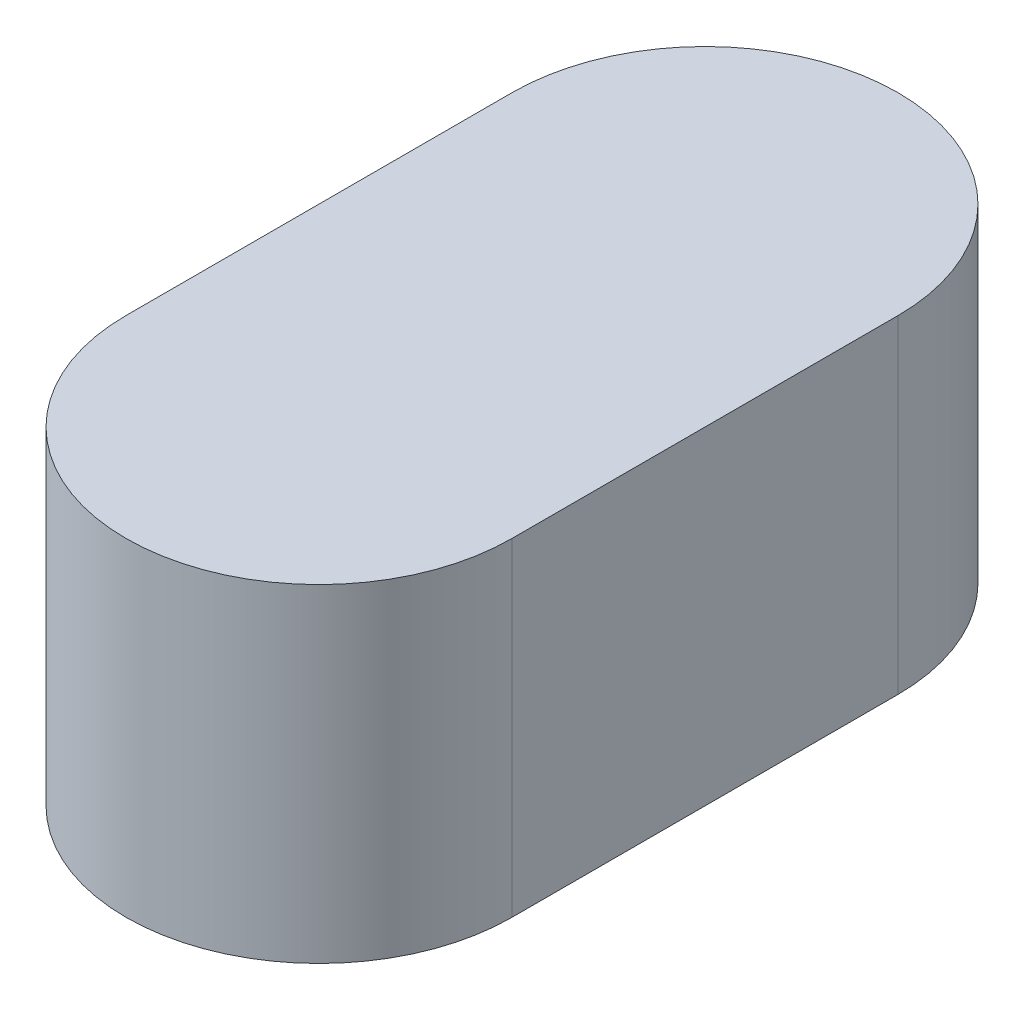
SolidWorks part; units mm, degrees
ref_plane "Front Plane" through (0, 0, 0) normal (0, 0, 1) x (1, 0, 0)
ref_plane "Top Plane" through (0, 0, 0) normal (0, 1, 0) x (1, 0, 0)
ref_plane "Right Plane" through (0, 0, 0) normal (1, 0, 0) x (0, 0, -1)
sketch "Sketch1" plane through (0, 0, 0) normal (0, 1, 0) x (1, 0, 0)
  line L0 (0, 46.6621) -> (0, -43.088) construction
  line L1 (-5, 5) -> (-5, -5)
  line L2 (5, -5) -> (5, 5)
  line L3 (-12.8752, 0) -> (12.7179, 0) construction
  arc A0 (-5, -5) -> (5, -5) centre (0, -5) ccw
  arc A1 (5, 5) -> (-5, 5) centre (0, 5) ccw
  dimension "D1" = 10
  dimension "D2" = 10
extrude "Boss-Extrude1" add sketch "Sketch1" along normal blind 8.5
